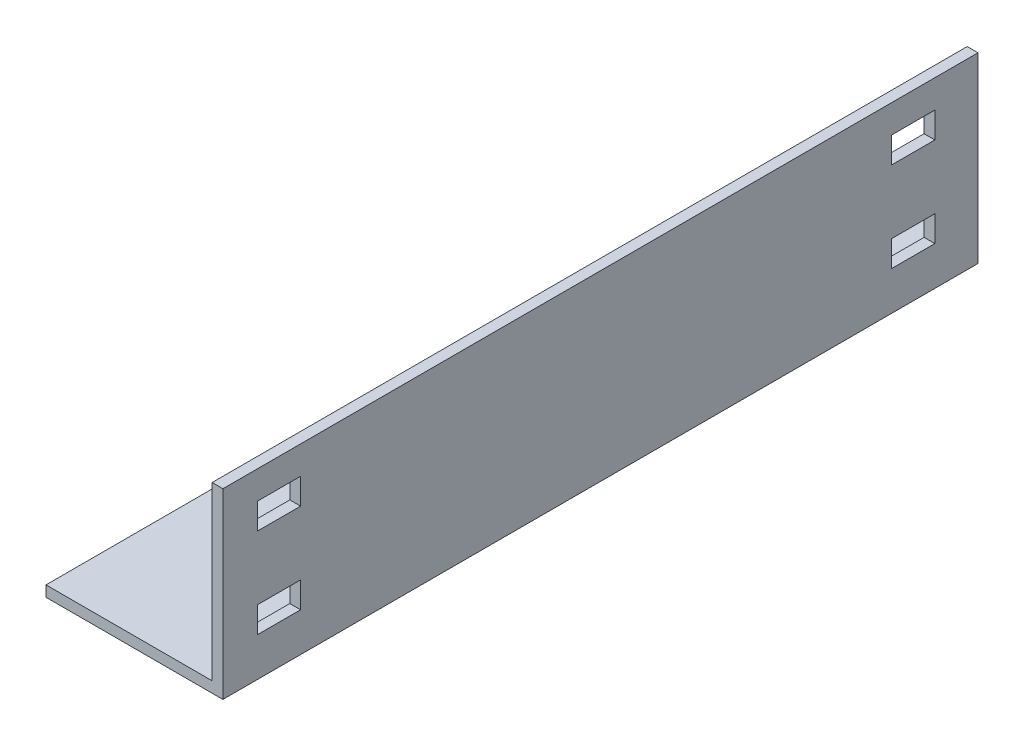
from build123d import *

# Parameters (mm, degrees)
EXTRUDE_1_DEPTH     = 875
SKETCH_2_W          = 100
SKETCH_2_H          = 60
CUT_EXTRUDE_2_DEPTH = 1017.542118193


with BuildPart() as part:
    # 草图1 → 凸台-拉伸1 (new, symmetric)
    with BuildSketch(Plane.XY):
        Polygon((-295.14043786, 27.019055308), (-295.14043786, 2.019055308), (114.859562138, 2.019055308), (114.859562138, 425), (89.859562138, 425), (89.859562138, 27.019055308), align=None)
    extrude(amount=EXTRUDE_1_DEPTH, both=True)

    # 草图2 → 切除-拉伸2 (cut, through all)
    with BuildSketch(Plane(origin=(0, 0, 0), x_dir=(0, 0, -1), z_dir=(1, 0, 0))):
        with Locations((725, 330)):
            Rectangle(SKETCH_2_W, SKETCH_2_H)
        with Locations((-745, 330)):
            Rectangle(SKETCH_2_W, SKETCH_2_H)
        with Locations((725, 122.019055308)):
            Rectangle(SKETCH_2_W, SKETCH_2_H)
        with Locations((-745, 122.019055308)):
            Rectangle(SKETCH_2_W, SKETCH_2_H)
    extrude(amount=CUT_EXTRUDE_2_DEPTH, mode=Mode.SUBTRACT)


solid = part.part
